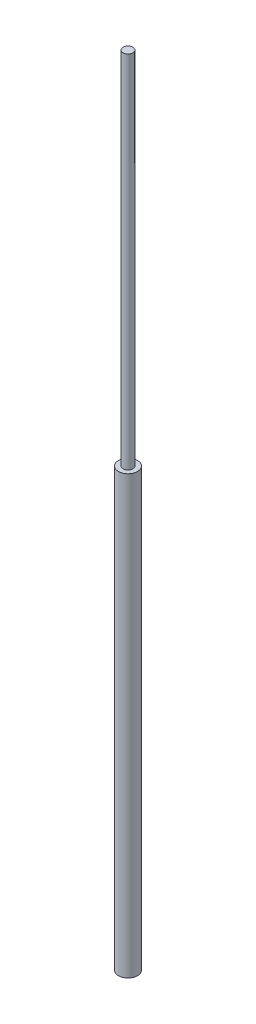
SolidWorks part; units mm, degrees
material "ABS"
ref_plane "Front Plane" through (0, 0, 0) normal (0, 0, 1) x (1, 0, 0)
ref_plane "Top Plane" through (0, 0, 0) normal (0, 1, 0) x (1, 0, 0)
ref_plane "Right Plane" through (0, 0, 0) normal (1, 0, 0) x (0, 0, -1)
sketch "Sketch1" plane through (0, 0, 0) normal (0, 1, 0) x (1, 0, 0)
  circle A0 centre (0, 0) radius 0.875
  dimension "D1" = 1.75
extrude "Boss-Extrude1" add sketch "Sketch1" along normal blind 40
sketch "Sketch2" plane through (0, 40, 0) normal (0, 1, 0) x (1, 0, 0)
  circle A0 centre (0, 0) radius 0.45
  dimension "D1" = 0.9
extrude "Boss-Extrude2" add sketch "Sketch2" along normal blind 33
